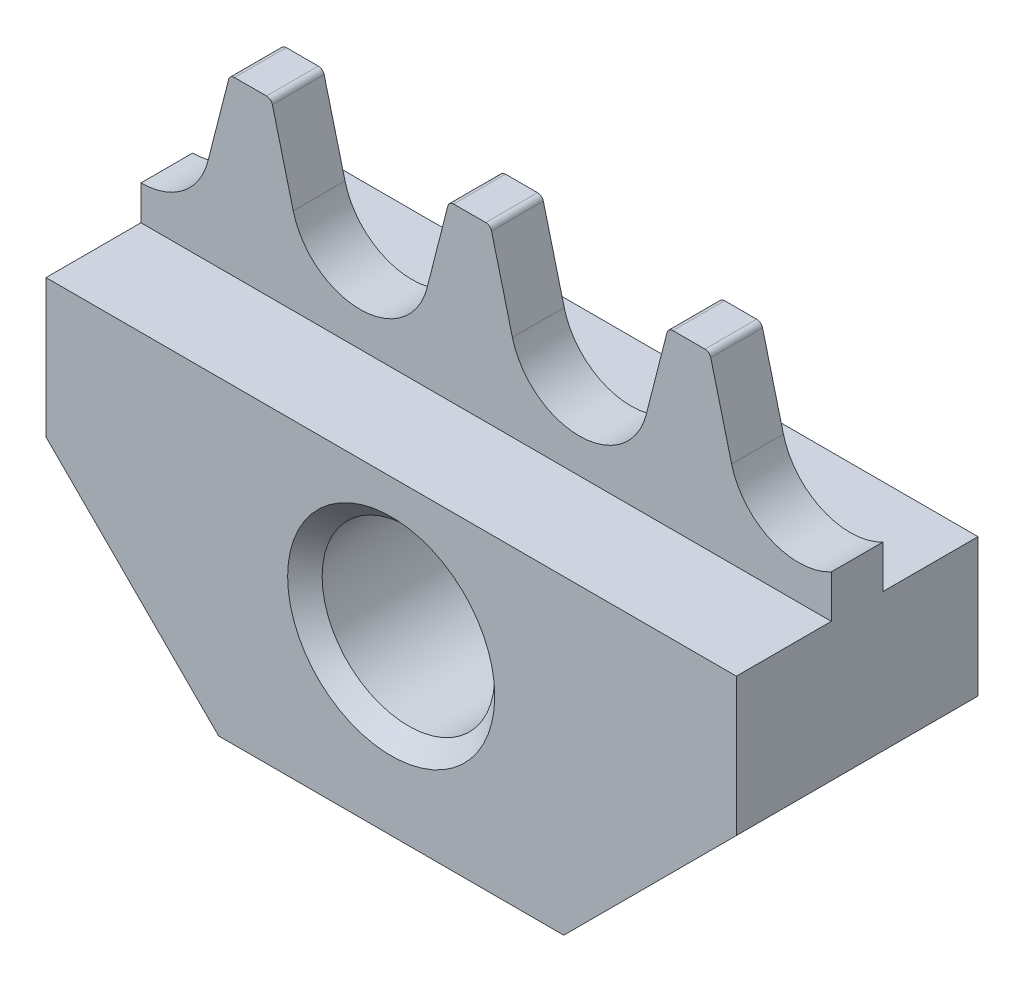
from build123d import *

# Parameters (mm, degrees)
SKETCH_1_R      = 5
EXTRUDE_1_DEPTH = 7
EXTRUDE_2_DEPTH = 1.5
FILLET_1_R      = 0.35
CHAMFER_1_SIZE  = 1


with BuildPart() as part:
    # 草图1 → 凸台-拉伸1 (new, symmetric)
    with BuildSketch(Plane.XY):
        Polygon((20, 18), (-20, 18), (-20, 10), (-10, 0), (10, 0), (20, 10), align=None)
        with Locations((0, 10)):
            Circle(SKETCH_1_R, mode=Mode.SUBTRACT)
    extrude(amount=EXTRUDE_1_DEPTH, both=True)

    # 草图2 → 凸台-拉伸2 (add, symmetric)
    with BuildSketch(Plane.XY):
        with BuildLine():
            Line((-14.85, 28), (-12.45, 28))
            Line((-12.45, 28), (-11.175595273, 23.010171086))
            ThreePointArc((-11.175595273, 23.010171086), (-7.3, 20), (-3.424404727, 23.010171086))
            Line((-3.424404727, 23.010171086), (-2.15, 28))
            Line((-2.15, 28), (0.25, 28))
            Line((0.25, 28), (1.524404727, 23.010171086))
            ThreePointArc((1.524404727, 23.010171086), (5.4, 20), (9.275595273, 23.010171086))
            Line((9.275595273, 23.010171086), (10.55, 28))
            Line((10.55, 28), (12.95, 28))
            Line((12.95, 28), (14.224404727, 23.010171086))
            ThreePointArc((14.224404727, 23.010171086), (16.494972361, 20.336137792), (20, 20.480056819))
            Line((20, 20.480056819), (20, 18))
            Line((20, 18), (-20, 18))
            Line((-20, 18), (-20, 20))
            ThreePointArc((-20, 20), (-17.546361442, 20.840940357), (-16.124404727, 23.010171086))
            Line((-16.124404727, 23.010171086), (-14.85, 28))
        make_face()
    extrude(amount=EXTRUDE_2_DEPTH, both=True)

    # 圆角1
    fillet_1_edges = [part.edges().sort_by_distance(p)[0] for p in [
        (12.95, 28, 0),
        (10.55, 28, 0),
        (0.25, 28, 0),
        (-2.15, 28, 0),
        (-12.45, 28, 0),
        (-14.85, 28, 0),
    ]]
    fillet(fillet_1_edges, radius=FILLET_1_R)

    # 倒角1
    chamfer_1_edges = [part.edges().sort_by_distance(p)[0] for p in [
        (-5, 10, -7),
        (-5, 10, 7),
    ]]
    chamfer(chamfer_1_edges, length=CHAMFER_1_SIZE)


solid = part.part
